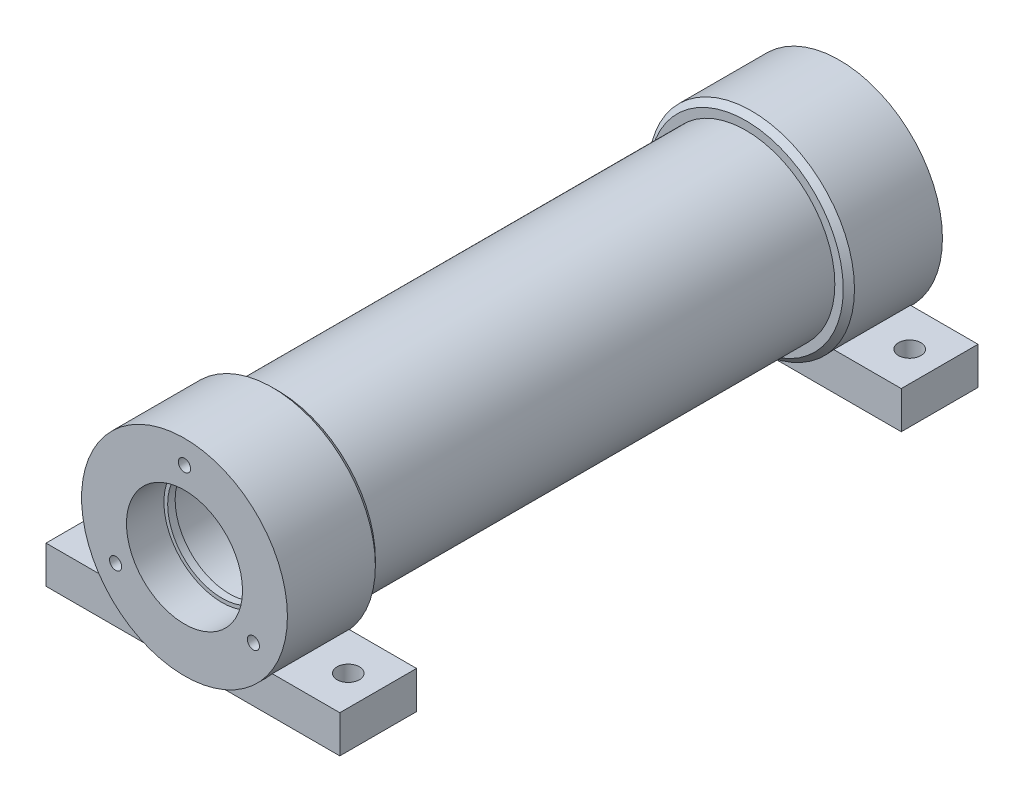
SolidWorks part; units mm, degrees
material "普通碳钢"
ref_plane "Front Plane" through (0, 0, 0) normal (0, 0, 1) x (1, 0, 0)
ref_plane "Top Plane" through (0, 0, 0) normal (0, 1, 0) x (1, 0, 0)
ref_plane "Right Plane" through (0, 0, 0) normal (1, 0, 0) x (0, 0, -1)
sketch "Sketch1" plane through (0, 0, 0) normal (0, 0, 1) x (1, 0, 0)
  circle A0 centre (0, 0) radius 55
  circle A1 centre (0, 0) radius 29
  dimension "D1" = 110
  dimension "D2" = 58
extrude "Boss-Extrude1" add sketch "Sketch1" along normal blind 350
ref_plane "Plane1" through (0, -55, 0) normal (0, 1, 0) x (1, 0, 0)
sketch "Sketch3" plane through (0, -55, 0) normal (0, 1, 0) x (1, 0, 0)
  line L0 (78.5, -45.5) -> (78.5, -304.5) construction
  line L1 (78.5, -4.5) -> (-78.5, -4.5)
  line L2 (78.5, -4.5) -> (78.5, -45.5)
  line L3 (78.5, -45.5) -> (-78.5, -45.5)
  line L4 (-78.5, -4.5) -> (-78.5, -45.5)
  line L5 (78.5, -4.5) -> (-78.5, -45.5) construction
  line L6 (78.5, -45.5) -> (-78.5, -4.5) construction
  line L7 (78.5, -304.5) -> (-78.5, -304.5)
  line L8 (78.5, -304.5) -> (78.5, -345.5)
  line L9 (78.5, -345.5) -> (-78.5, -345.5)
  line L10 (-78.5, -304.5) -> (-78.5, -345.5)
  line L11 (78.5, -304.5) -> (-78.5, -345.5) construction
  line L12 (78.5, -345.5) -> (-78.5, -304.5) construction
  line L13 (55, -350) -> (55, 0) construction
  line L14 (55, -350) -> (55, 0) construction
  line L15 (62.5, -25) -> (-62.5, -25) construction
  line L16 (55, 0) -> (-55, 0) construction
  line L17 (55, 0) -> (-55, 0) construction
  circle A0 centre (62.5, -25) radius 6
  circle A1 centre (62.5, -325) radius 6
  circle A2 centre (-62.5, -25) radius 6
  circle A3 centre (-62.5, -325) radius 6
  point P4 (0, -25)
  point P9 (0, -325)
  point P12 (78.5, -175)
  point P13 (55, -175)
  point P22 (0, -25)
  point P25 (0, 0)
  dimension "D2" = 12
  dimension "D1" = 341
  dimension "D3" = 125
  dimension "D4" = 157
  dimension "D5" = 300
extrude "Boss-Extrude2" add sketch "Sketch3" along normal blind 20 contours L1 L4 L3 L2 A2 A0 | L7 L10 L9 L8 A3 A1
ref_plane "Plane2" through (0, 0, 330) normal (0, 0, 1) x (1, 0, 0)
sketch "Sketch6" plane through (0, 0, 330) normal (0, 0, 1) x (1, 0, 0)
  circle A0 centre (0, 0) radius 31
  circle A1 centre (0, 0) radius 29 construction
  circle A2 centre (0, 0) radius 29
  dimension "D1" = 62
extrude "Cut-Extrude1" cut sketch "Sketch6" along normal through all
ref_plane "Plane3" through (0, 0, 20) normal (0, 0, -1) x (-1, 0, 0)
sketch "Sketch8" plane through (0, 0, 0) normal (0, 0, -1) x (-1, 0, 0)
  circle A0 centre (0, 0) radius 31
  dimension "D1" = 62
extrude "Cut-Extrude2" cut sketch "Sketch8" against normal blind 306 from offset 20 offset against normal yes
sketch "Sketch9" plane through (0, 0, 0) normal (0, 0, -1) x (-1, 0, 0)
  circle A0 centre (0, 0) radius 36
  dimension "D1" = 72
extrude "Cut-Extrude3" cut sketch "Sketch9" against normal blind 21
sketch "Sketch10" plane through (0, -55, 0) normal (0, -1, 0) x (1, 0, 0)
  text T0 "前"
extrude "Cut-Extrude4" cut sketch "Sketch10" against normal blind 5
sketch "Sketch12" plane through (0, 0, 0) normal (0, 0, -1) x (-1, 0, 0)
  line L0 (0, 42.5) -> (0, 0) construction
  line L1 (0, 0) -> (-36.8061, -21.25) construction
  line L2 (0, 0) -> (36.8061, -21.25) construction
  circle A0 centre (0, 0) radius 42.5 construction
  circle A1 centre (0, 42.5) radius 3.25
  circle A2 centre (-36.8061, -21.25) radius 3.25
  circle A3 centre (36.8061, -21.25) radius 3.25
  dimension "D3" = 85
  dimension "D4" = 6.5
  dimension "D1" = 120
  dimension "D2" = 120
extrude "Cut-Extrude5" cut sketch "Sketch12" against normal blind 5
sketch "Sketch13" plane through (0, 0, 350) normal (0, 0, 1) x (1, 0, 0)
  line L0 (0, 42.5) -> (0, 0) construction
  line L1 (0, 0) -> (-36.8061, -21.25) construction
  line L2 (0, 0) -> (36.8061, -21.25) construction
  circle A0 centre (0, 0) radius 42.5 construction
  circle A1 centre (0, 42.5) radius 3.25
  circle A2 centre (-36.8061, -21.25) radius 3.25
  circle A3 centre (36.8061, -21.25) radius 3.25
  dimension "D1" = 85
  dimension "D2" = 6.5
  dimension "D3" = 120
  dimension "D4" = 120
extrude "Cut-Extrude6" cut sketch "Sketch13" against normal blind 5
sketch "Sketch14" plane through (0, 0, 350) normal (0, 0, 1) x (1, 0, 0)
  circle A0 centre (0, 0) radius 47.5
  circle A1 centre (0, 0) radius 55 construction
  circle A2 centre (0, 0) radius 55
  dimension "D1" = 95
extrude "Cut-Extrude7" cut sketch "Sketch14" against normal blind 250 from offset 50 offset against normal yes
chamfer "Chamfer1" distance 3 angle 45 2 edges at (55, 0, 50) (55, 0, 300)
